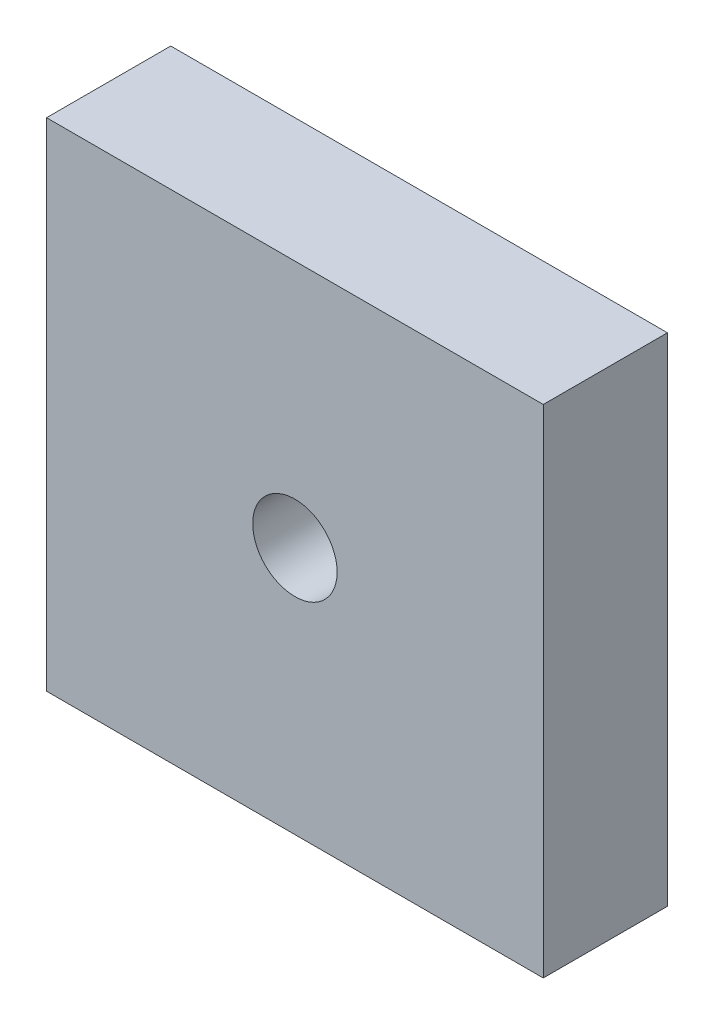
from build123d import *

# Parameters (mm, degrees)
SKETCH_1_W         = 40
SKETCH_1_H         = 40
EXTRUDE_1_DEPTH    = 5
HOLE_WIZARD_M8_1_D = 6.8


with BuildPart() as part:
    # 草图1 → 凸台-拉伸1 (new, symmetric)
    with BuildSketch(Plane.XY):
        Rectangle(SKETCH_1_W, SKETCH_1_H)
    extrude(amount=EXTRUDE_1_DEPTH, both=True)

    # M8 螺纹孔1 (through all)
    with Locations(Plane.XY.offset(5)):
        with Locations((0, 0)):
            Hole(HOLE_WIZARD_M8_1_D / 2)


solid = part.part
